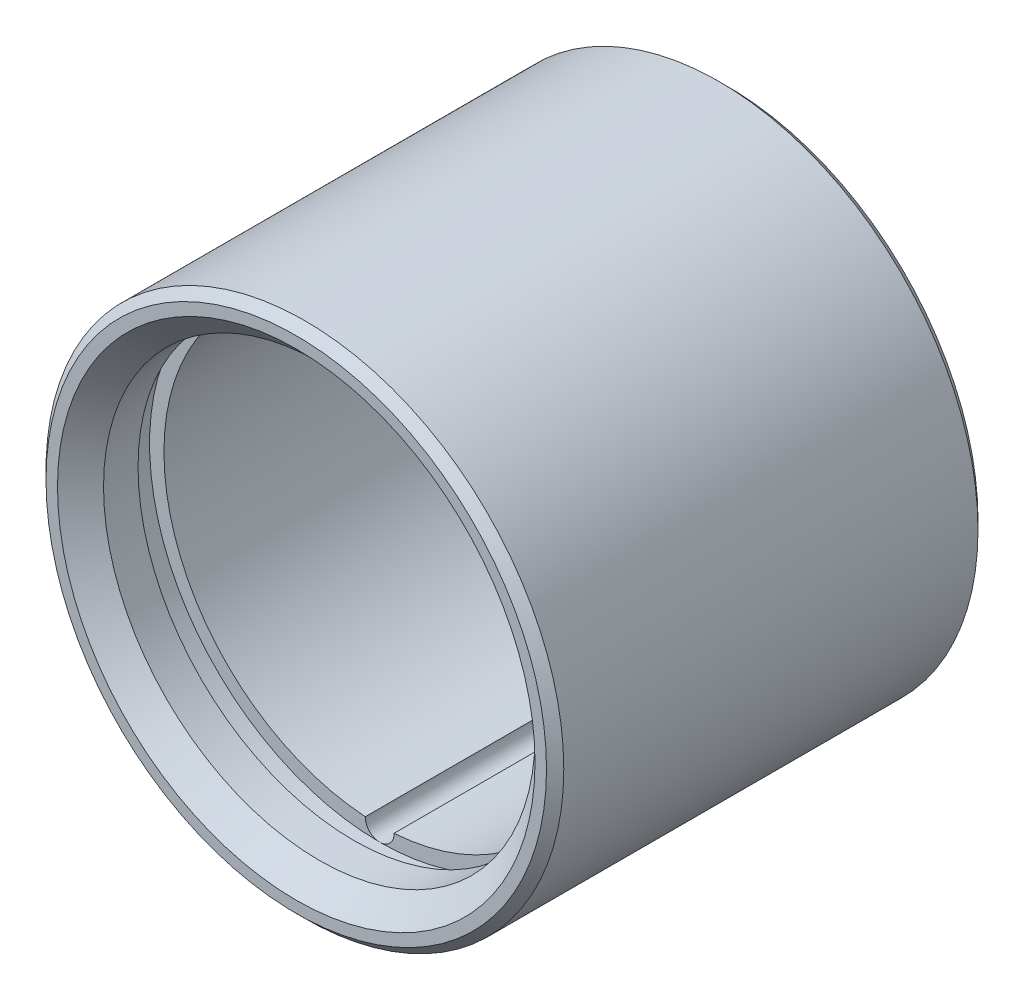
SolidWorks part; units mm, degrees
material "ZCuSn10Pb5"
ref_plane "Front Plane" through (0, 0, 0) normal (0, 0, 1) x (1, 0, 0)
ref_plane "Top Plane" through (0, 0, 0) normal (0, 1, 0) x (1, 0, 0)
ref_plane "Right Plane" through (0, 0, 0) normal (1, 0, 0) x (0, 0, -1)
sketch "Sketch1" plane through (0, 0, 0) normal (0, 0, 1) x (1, 0, 0)
  circle A0 centre (0, 0) radius 37.5
  circle A1 centre (0, 0) radius 45
  dimension "D1" = 75
  dimension "D2" = 90
extrude "Boss-Extrude1" add sketch "Sketch1" along normal mid plane 75
ref_plane "Plane1" through (0, 0, 27.5) normal (0, 0, 1) x (1, 0, 0)
sketch "Sketch2" plane through (0, 0, 27.5) normal (0, 0, 1) x (1, 0, 0)
  circle A0 centre (0, 0) radius 40
  circle A1 centre (0, 0) radius 37.5 construction
  circle A2 centre (0, 0) radius 37.5
  dimension "D1" = 80
extrude "Cut-Extrude1" cut sketch "Sketch2" against normal blind 4.5
chamfer "ChamferC1.5" distance 1.5 angle 45 3 edges at (37.5, 0, -37.5) (45, 0, -37.5) (45, 0, 37.5)
chamfer "ChamferC4" distance 4 angle 45 1 edges at (37.5, 0, 37.5)
sketch "Sketch3" plane through (0, 0, 27.5) normal (0, 0, 1) x (1, 0, 0)
  line L0 (0, 0) -> (0, -21.3095) construction
  line L1 (0, -40) -> (19.4249, -40) construction
  line L2 (-1.1597, -37.5) -> (18.2652, -37.5) construction
  line L3 (-0.7351, 0) -> (18.6898, 0) construction
  circle A0 centre (0, 0) radius 37.5 construction
  arc A1 (2.4986, 37.4167) -> (-2.4986, 37.4167) centre (0, 0) ccw
  arc A2 (-2.4986, -37.4167) -> (2.4986, -37.4167) centre (0, -37.5) ccw
  arc A3 (-2.4986, 37.4167) -> (2.4986, 37.4167) centre (0, 37.5) cw
  arc A4 (-2.4986, -37.4167) -> (2.4986, -37.4167) centre (0, 0) ccw
  dimension "D2" = 2.5
  dimension "D1" = 2.5
extrude "Cut-Extrude2" cut sketch "Sketch3" against normal through all
